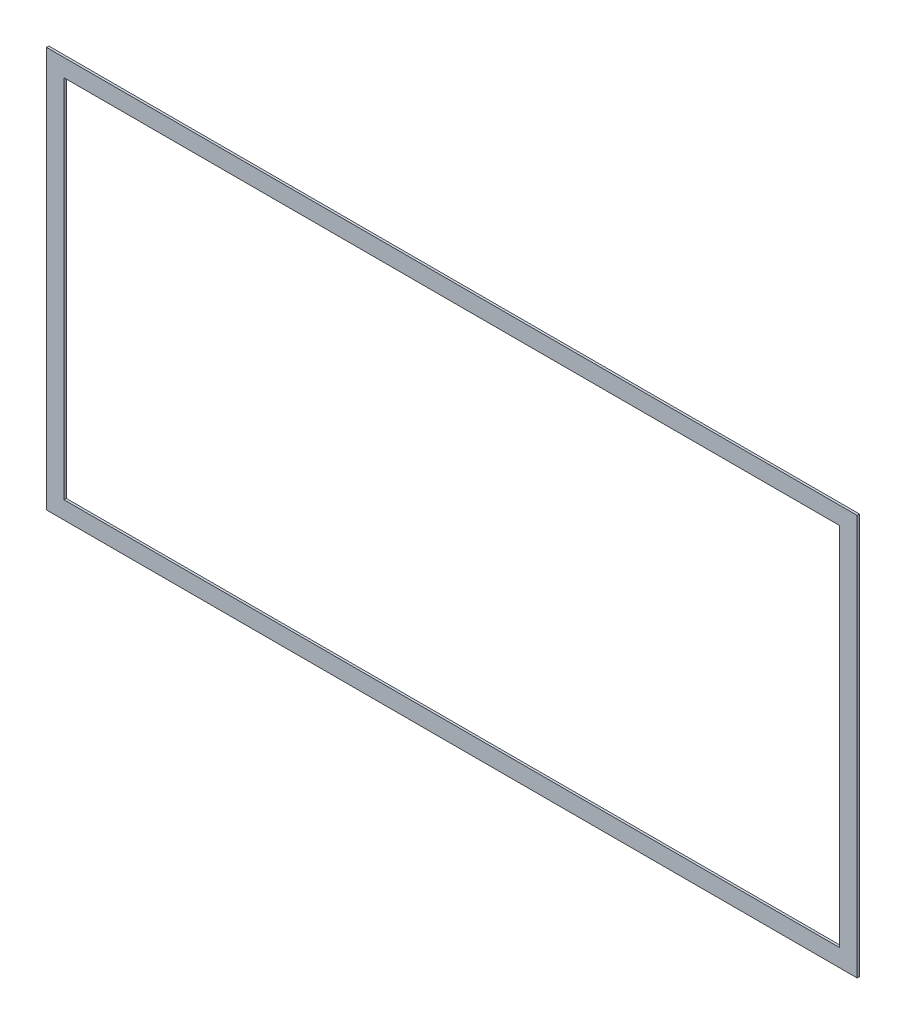
from build123d import *

# Parameters (mm, degrees)
SKETCH_1_W      = 692
SKETCH_1_H      = 342
SKETCH_1_W_2    = 662
SKETCH_1_H_2    = 312
EXTRUDE_1_DEPTH = 1


with BuildPart() as part:
    # 草图1 → 凸台-拉伸1 (new, symmetric)
    with BuildSketch(Plane.XY):
        Rectangle(SKETCH_1_W, SKETCH_1_H)
        Rectangle(SKETCH_1_W_2, SKETCH_1_H_2, mode=Mode.SUBTRACT)
    extrude(amount=EXTRUDE_1_DEPTH, both=True)


solid = part.part
